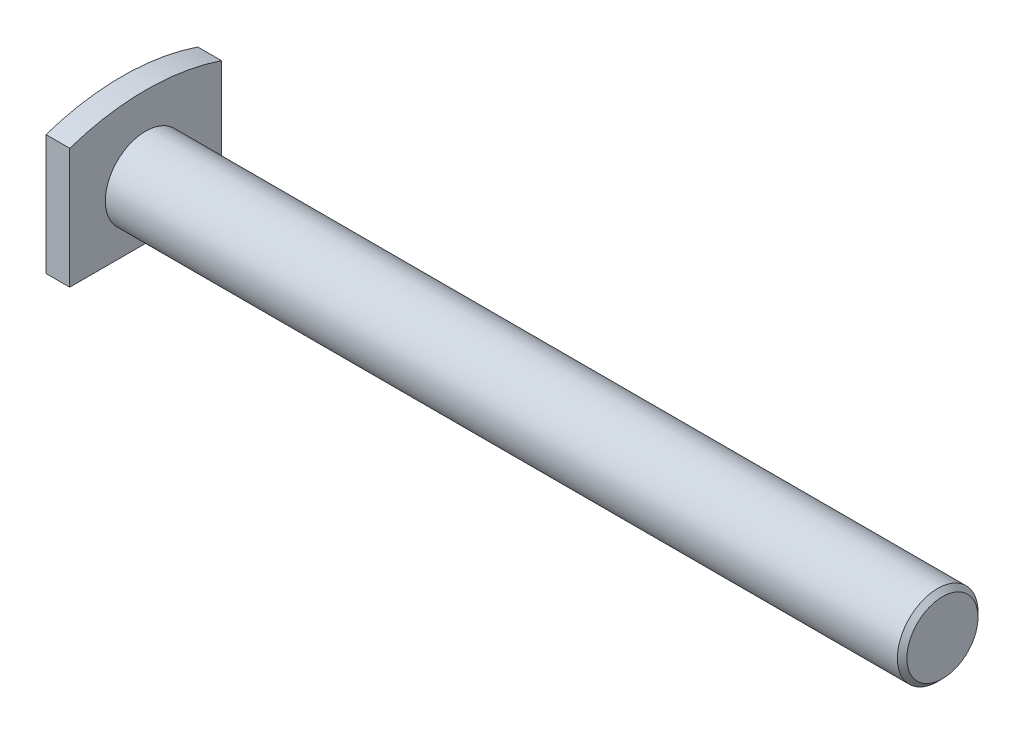
from build123d import *

# Parameters (mm, degrees)
SKETCH_1_W      = 84
SKETCH_1_H      = 4.25
CHAMFER_1_SIZE  = 0.5
EXTRUDE_1_DEPTH = 2.5


with BuildPart() as part:
    # 草图1 → 旋转1 (revolve)
    with BuildSketch(Plane.XY, mode=Mode.PRIVATE) as revolve_1_sk:
        with Locations((42, -2.125)):
            Rectangle(SKETCH_1_W, SKETCH_1_H)
    revolve(revolve_1_sk.sketch.rotate(Axis((-1.134146341, 0, 0), (1, 0, 0)), 270), axis=Axis((-1.134146341, 0, 0), (1, 0, 0)))

    # 倒角1
    chamfer_1_edges = [part.edges().sort_by_distance(p)[0] for p in [
        (84, 0, -4.25),
    ]]
    chamfer(chamfer_1_edges, length=CHAMFER_1_SIZE)

    # 草图2 → 凸台-拉伸1 (add)
    with BuildSketch(Plane.ZY):
        with BuildLine():
            Line((-8, 6.685438565), (-8, -6))
            Line((-8, -6), (8, -6))
            Line((8, -6), (8, 6.685438565))
            ThreePointArc((8, 6.685438565), (0, 8), (-8, 6.685438565))
        make_face()
    extrude(amount=EXTRUDE_1_DEPTH)


solid = part.part
